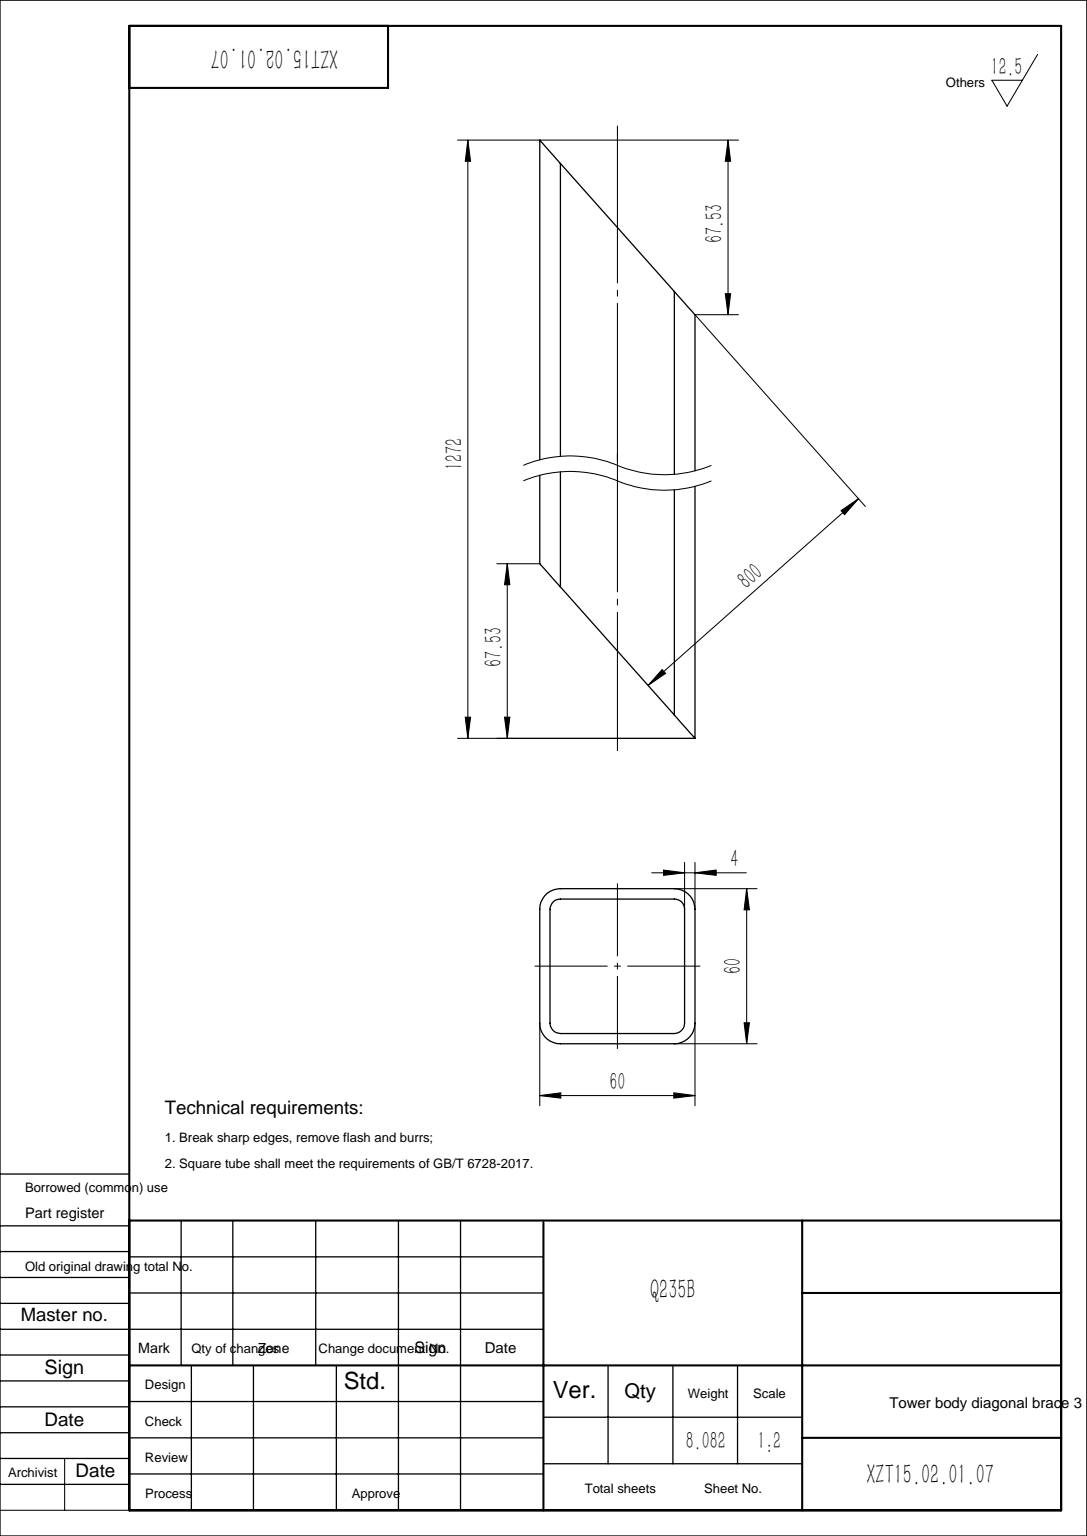
SolidWorks part; units mm, degrees
material "Q235B"
ref_plane "Front Plane" through (0, 0, 0) normal (0, 0, 1) x (1, 0, 0)
ref_plane "Top Plane" through (0, 0, 0) normal (0, 1, 0) x (1, 0, 0)
ref_plane "Right Plane" through (0, 0, 0) normal (1, 0, 0) x (0, 0, -1)
sketch "草图1" plane through (0, 0, 0) normal (0, 0, 1) x (1, 0, 0)
  line L0 (0, 0) -> (0, 1272)
  dimension "D1" = 1272
other "GB/T 6728-2002 square hollow section 60×60×4(1)"
ref_plane "Plane1" through (0, 0, 0) normal (0, 1, 0) x (-1, 0, 0)
sketch "Sketch1" plane through (0, 0, 0) normal (0, 1, 0) x (-1, 0, 0)
  line L0 (-22, -26) -> (22, -26)
  line L1 (-26, -22) -> (-26, 22)
  line L2 (22, 26) -> (-22, 26)
  line L3 (26, 22) -> (26, -22)
  line L4 (-22, -30) -> (22, -30)
  line L5 (-30, -22) -> (-30, 22)
  line L6 (22, 30) -> (-22, 30)
  line L7 (30, 22) -> (30, -22)
  arc A0 (30, 22) -> (22, 30) centre (22, 22) ccw
  arc A1 (22, -30) -> (30, -22) centre (22, -22) ccw
  arc A2 (-30, -22) -> (-22, -30) centre (-22, -22) ccw
  arc A3 (-22, 30) -> (-30, 22) centre (-22, 22) ccw
  arc A4 (-22, 26) -> (-26, 22) centre (-22, 22) ccw
  arc A5 (26, 22) -> (22, 26) centre (22, 22) ccw
  arc A6 (22, -26) -> (26, -22) centre (22, -22) ccw
  arc A7 (-26, -22) -> (-22, -26) centre (-22, -22) ccw
  point P0 (-30, 0)
  point P1 (30, 0)
  point P2 (0, 30)
  point P3 (0, -30)
  point P4 (0, 0)
  point P5 (-30, -30)
  point P6 (30, -30)
  point P7 (30, 30)
  point P8 (-30, 30)
  point P33 (0, 0)
  dimension "D1" = 8
  dimension "Thickness" = 4
  dimension "V_leg" = 60
sketch "Sketch2" plane through (0, 0, 30) normal (0, 0, 1) x (1, 0, 0)
  line L0 (-30, 1272) -> (30, 1204.4689)
  line L1 (30, 1272) -> (30, 0) construction
  line L2 (30, 1204.4689) -> (30, 1272)
  line L3 (30, 1272) -> (-30, 1272)
  line L4 (-30, 0) -> (-30, 67.5311)
  line L5 (-30, 1272) -> (-30, 0) construction
  line L6 (-30, 67.5311) -> (30, 0)
  line L7 (30, 0) -> (-30, 0)
  dimension "D1" = 800
extrude "Cut-Extrude1" cut sketch "Sketch2" against normal through all both and the other way through all
